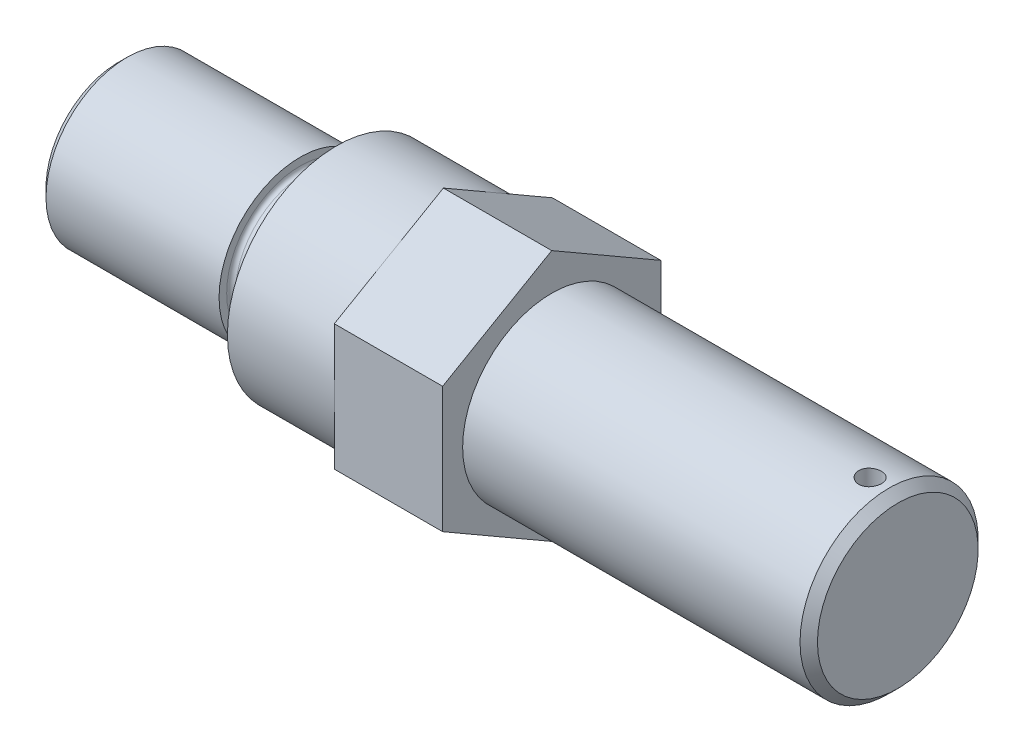
SolidWorks part; units mm, degrees
material "普通碳钢"
ref_plane "Front Plane" through (0, 0, 0) normal (0, 0, 1) x (1, 0, 0)
ref_plane "Top Plane" through (0, 0, 0) normal (0, 1, 0) x (1, 0, 0)
ref_plane "Right Plane" through (0, 0, 0) normal (1, 0, 0) x (0, 0, -1)
sketch "Sketch1" plane through (0, 0, 0) normal (0, 0, 1) x (1, 0, 0)
  line L0 (0, 0) -> (87.6275, 0) construction
  line L1 (0, 0) -> (0, 83.708) construction
  line L2 (0, 0) -> (0, 14.1605)
  line L3 (0, 14.1605) -> (31.75, 14.1605)
  line L4 (31.75, 14.1605) -> (31.75, 12.065)
  line L5 (31.75, 12.065) -> (38.1, 12.065)
  line L6 (38.1, 12.065) -> (38.1, 19.05)
  line L7 (38.1, 19.05) -> (75.692, 19.05)
  line L8 (75.692, 19.05) -> (75.692, 15.5575)
  line L9 (75.692, 15.5575) -> (136.144, 15.5575)
  line L10 (136.144, 15.5575) -> (136.144, 0)
  line L11 (0, 0) -> (136.144, 0)
  dimension "D1" = 19.05
  dimension "D2" = 14.1605
  dimension "D3" = 12.065
  dimension "D4" = 60.452
  dimension "D5" = 136.144
  dimension "D6" = 98.044
  dimension "D7" = 31.75
revolve "Revolve1" add sketch "Sketch1" angle 360 about L11
chamfer "Chamfer1" distance 1.524 angle 45 2 edges at (0, 0, 14.1605) (136.144, 0, 15.5575)
sketch "Sketch2" plane through (75.692, 0, 0) normal (1, 0, 0) x (0, 0, -1)
  line L1 (0, 21.997) -> (-19.05, 10.9985)
  line L2 (-19.05, 10.9985) -> (-19.05, -10.9985)
  line L3 (-19.05, -10.9985) -> (0, -21.997)
  line L4 (0, -21.997) -> (19.05, -10.9985)
  line L5 (19.05, -10.9985) -> (19.05, 10.9985)
  line L6 (19.05, 10.9985) -> (0, 21.997)
  circle A0 centre (0, 0) radius 19.05 construction
  circle A1 centre (0, 0) radius 19.05 construction
extrude "Boss-Extrude1" add sketch "Sketch2" against normal blind 18.923
fillet "Fillet1" radius 0.762 2 edges at (31.75, 0, 12.065) (38.1, 0, 12.065)
sketch "Sketch3" plane through (0, 0, 0) normal (0, 1, 0) x (1, 0, 0)
  line L0 (136.144, -14.0335) -> (136.144, 14.0335) construction
  circle A0 centre (131.318, 0) radius 1.9844
  dimension "D1" = 3.9687
  dimension "D2" = 4.826
extrude "Cut-Extrude1" cut sketch "Sketch3" against normal mid plane 50
